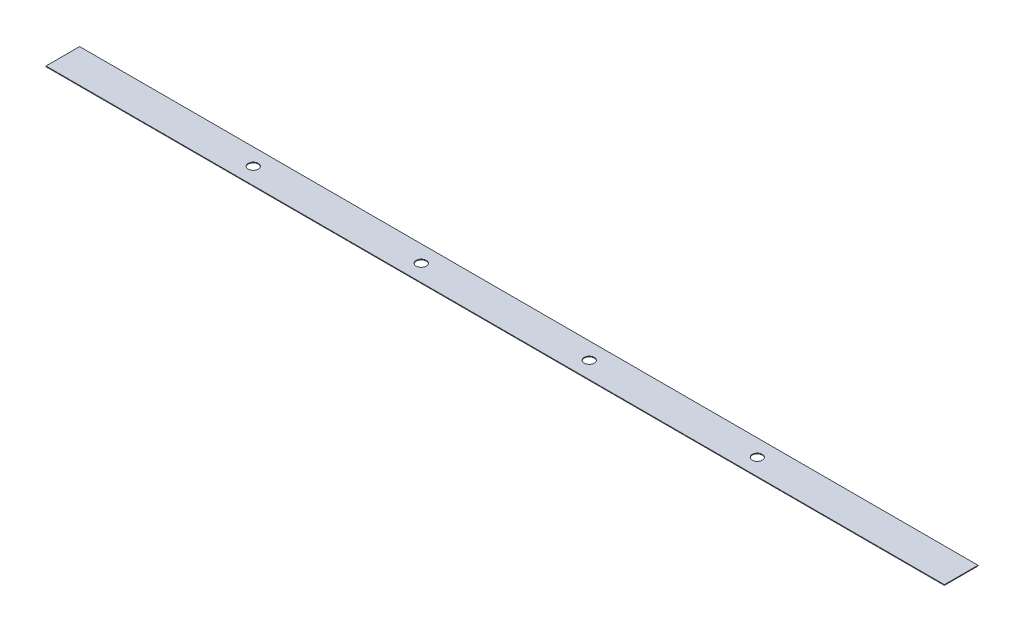
from build123d import *

# Parameters (mm, degrees)
SKETCH1_W           = 16040
SKETCH1_H           = 600
BOSS_EXTRUDE1_DEPTH = 12
SKETCH2_R           = 90
CUT_EXTRUDE1_DEPTH  = 8026.617982436
LPATTERN1_COUNT     = 4
LPATTERN1_PITCH     = 3000


with BuildPart() as part:
    # Sketch1 → Boss-Extrude1 (new body)
    with BuildSketch(Plane(origin=(0, 0, 0), x_dir=(1, 0, 0), z_dir=(0, 1, 0))):
        Rectangle(SKETCH1_W, SKETCH1_H)
    extrude(amount=BOSS_EXTRUDE1_DEPTH)

    # Sketch2 → Cut-Extrude1 (cut, through all)
    with BuildSketch(Plane(origin=(0, 12, 0), x_dir=(1, 0, 0), z_dir=(0, 1, 0))):
        with Locations(Location((-4620, 0, 0), (0, 0, 270))):
            Circle(SKETCH2_R)
    cut_extrude1 = extrude(amount=-CUT_EXTRUDE1_DEPTH, mode=Mode.SUBTRACT)

    # LPattern1: Cut-Extrude1 ×4
    with Locations(*[(i * LPATTERN1_PITCH, 0, 0) for i in range(1, LPATTERN1_COUNT)]):
        add(cut_extrude1, mode=Mode.SUBTRACT)


solid = part.part
